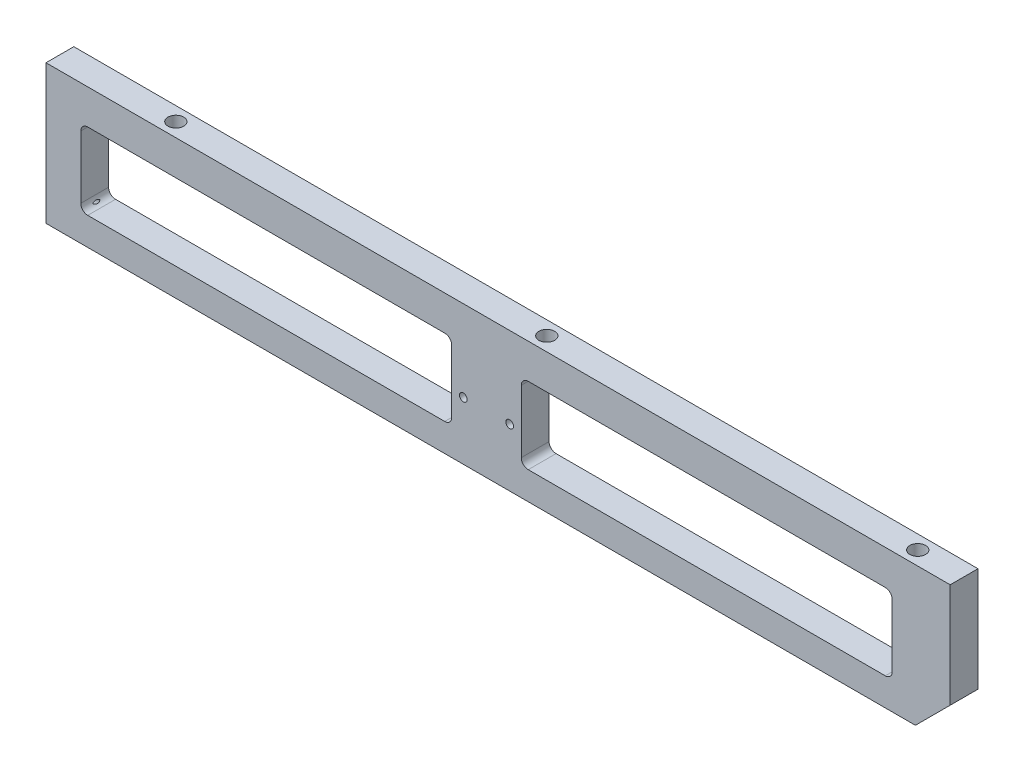
from build123d import *

# Parameters (mm, degrees)
EXTRUDE_1_DEPTH        = 6
HOLE_WIZARD_M8_1_D     = 6.8
HOLE_WIZARD_M8_1_DEPTH = 15.75
HOLE_WIZARD_M8_1_TIP   = 2.042926105
HOLE_WIZARD_M4_1_D     = 3.3
PATTERN_LINEAR_1_COUNT = 3
PATTERN_LINEAR_1_PITCH = 160


with BuildPart() as part:
    # 草图1 → 凸台-拉伸1 (new, symmetric)
    with BuildSketch(Plane.XY):
        Polygon((180, -30), (195, -15), (195, 30), (-195, 30), (-195, -30), align=None)
        with BuildLine():
            Line((-177, 15), (-23, 15))
            ThreePointArc((-23, 15), (-20.878679656, 14.121320344), (-20, 12))
            Line((-20, 12), (-20, -15))
            ThreePointArc((-20, -15), (-20.878679656, -17.121320344), (-23, -18))
            Line((-23, -18), (-177, -18))
            ThreePointArc((-177, -18), (-179.121320344, -17.121320344), (-180, -15))
            Line((-180, -15), (-180, 12))
            ThreePointArc((-180, 12), (-179.121320344, 14.121320344), (-177, 15))
        make_face(mode=Mode.SUBTRACT)
        with BuildLine():
            Line((13, 15), (167, 15))
            ThreePointArc((167, 15), (169.121320344, 14.121320344), (170, 12))
            Line((170, 12), (170, -15))
            ThreePointArc((170, -15), (169.121320344, -17.121320344), (167, -18))
            Line((167, -18), (13, -18))
            ThreePointArc((13, -18), (10.878679656, -17.121320344), (10, -15))
            Line((10, -15), (10, 12))
            ThreePointArc((10, 12), (10.878679656, 14.121320344), (13, 15))
        make_face(mode=Mode.SUBTRACT)
    extrude(amount=EXTRUDE_1_DEPTH, both=True)

    # M8 螺纹孔1
    with Locations(Plane(origin=(-195, 20, 0), x_dir=(0, 0, -1), z_dir=(-1, 0, 0))):
        with Locations((0, 0), (0, 40)):
            Hole(HOLE_WIZARD_M8_1_D / 2, depth=HOLE_WIZARD_M8_1_DEPTH)
            with Locations((0, 0, -(HOLE_WIZARD_M8_1_DEPTH + HOLE_WIZARD_M8_1_TIP / 2))):  # 118° drill point
                Cone(0, HOLE_WIZARD_M8_1_D / 2, HOLE_WIZARD_M8_1_TIP, mode=Mode.SUBTRACT)

    # M4 螺纹孔1 (through all)
    with Locations(Plane.XY.offset(6)):
        with Locations((-15, -5), (5, -5)):
            Hole(HOLE_WIZARD_M4_1_D / 2)

    # 草图6 → M8 螺纹孔2 (revolve, cut)
    with BuildSketch(Plane(origin=(-145, 30, 0), x_dir=(0, 0, 1), z_dir=(1, 0, 0))):
        Polygon((0, 0), (0, 17.792926105), (3.4, 15.75), (3.4, 0), align=None)
    hole_wizard_m8_2 = revolve(axis=Axis((-145, 36.35, 0), (0, -1, 0)), mode=Mode.SUBTRACT)

    # 阵列(线性)1: M8 螺纹孔2 ×3
    with Locations(*[(i * PATTERN_LINEAR_1_PITCH, 0, 0) for i in range(1, PATTERN_LINEAR_1_COUNT)]):
        add(hole_wizard_m8_2, mode=Mode.SUBTRACT)


solid = part.part
